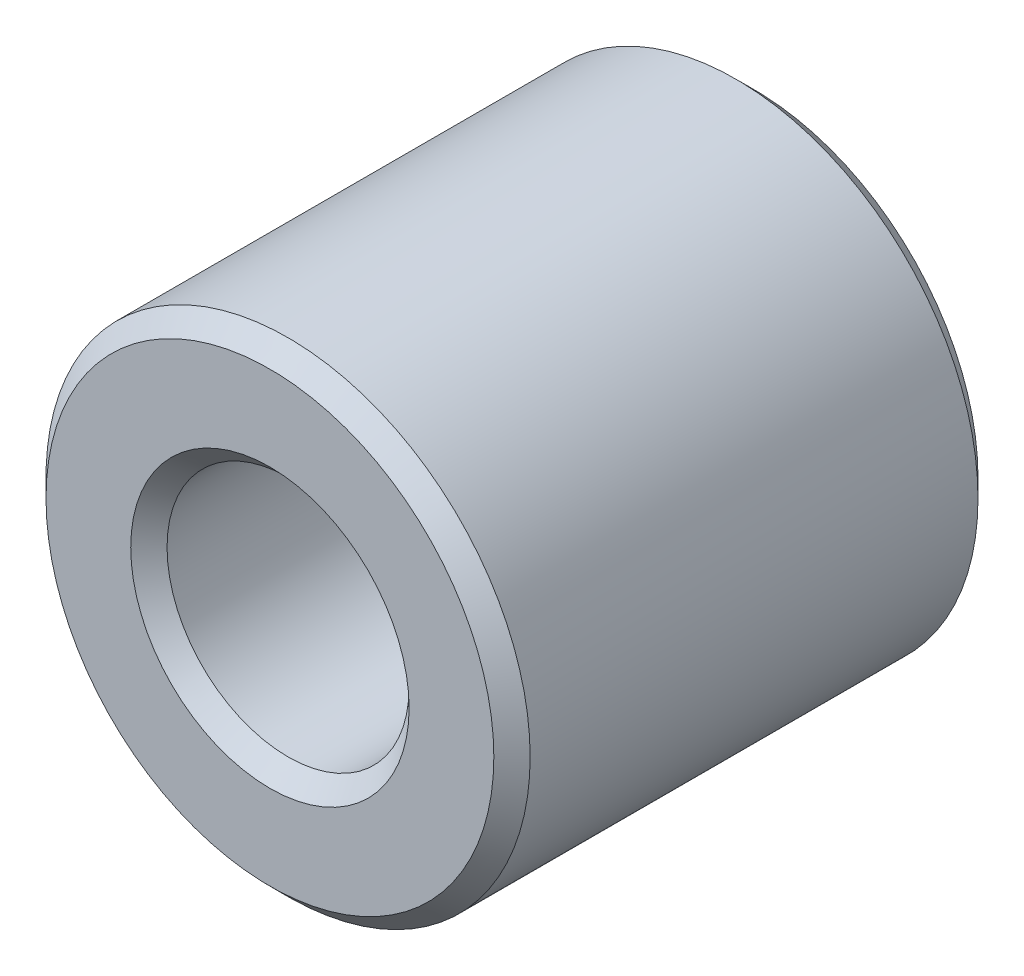
from build123d import *

# Parameters (mm, degrees)
SKETCH1_R           = 4
SKETCH1_R_2         = 2
BOSS_EXTRUDE1_DEPTH = 8
CHAMFER1_SIZE       = 0.3


with BuildPart() as part:
    # Sketch1 → Boss-Extrude1 (new body)
    with BuildSketch(Plane.XY):
        Circle(SKETCH1_R)
        Circle(SKETCH1_R_2, mode=Mode.SUBTRACT)
    extrude(amount=BOSS_EXTRUDE1_DEPTH)

    # Chamfer1
    chamfer1_edges = [part.edges().sort_by_distance(p)[0] for p in [
        (-4, 0, 0),
        (-4, 0, 8),
        (-2, 0, 0),
        (-2, 0, 8),
    ]]
    chamfer(chamfer1_edges, length=CHAMFER1_SIZE)


solid = part.part
